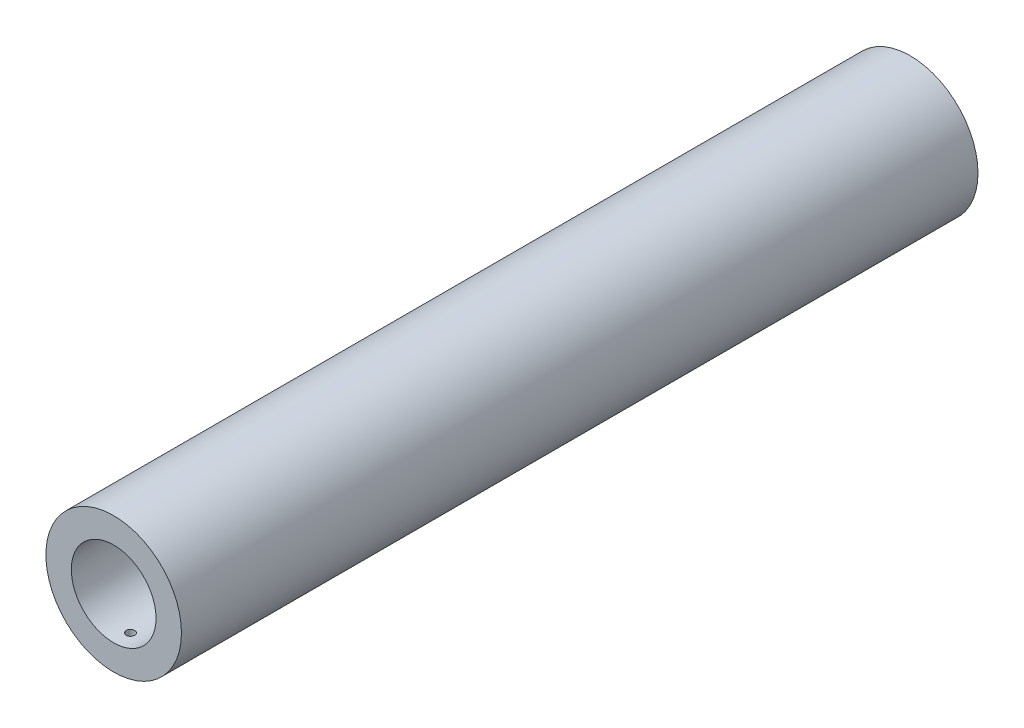
from build123d import *

# Parameters (mm, degrees)
SKETCH1_R               = 40
SKETCH1_R_2             = 25
BOSS_EXTRUDE1_DEPTH     = 470
CUT_EXTRUDE1_REACH      = 475.392
CUT_EXTRUDE1_END_RADIUS = 40
SKETCH2_R               = 2.5


with BuildPart() as part:
    # Sketch1 → Boss-Extrude1 (new body)
    with BuildSketch(Plane.XY):
        with Locations(Location((0, 0, 0), (0, 0, 180))):
            Circle(SKETCH1_R)
        with Locations(Location((0, 0, 0), (0, 0, 180))):
            Circle(SKETCH1_R_2, mode=Mode.SUBTRACT)
    extrude(amount=BOSS_EXTRUDE1_DEPTH)

    # Cut-Extrude1: up to this cylinder (the profile starts inside it)
    cut_extrude1_end = Plane(origin=(0, 0, 235), z_dir=(0, 0, -1)) * Cylinder(CUT_EXTRUDE1_END_RADIUS, 1481.784, mode=Mode.PRIVATE)
    # Sketch2 → Cut-Extrude1 (cut, up to the surface)
    with BuildSketch(Plane(origin=(0, 0, 0), x_dir=(1, 0, 0), z_dir=(0, 1, 0)), mode=Mode.PRIVATE) as cut_extrude1_sk1:
        with Locations(Location((0, -460, 0), (0, 0, 270))):
            Circle(SKETCH2_R)
    cut_extrude1_tool1 = extrude(cut_extrude1_sk1.sketch, amount=-CUT_EXTRUDE1_REACH, mode=Mode.PRIVATE) & cut_extrude1_end
    add(cut_extrude1_tool1.solids().sort_by_distance((0, 0, 460))[0], mode=Mode.SUBTRACT)
    # Sketch2 → Cut-Extrude1 (cut, up to the surface)
    with BuildSketch(Plane(origin=(0, 0, 0), x_dir=(1, 0, 0), z_dir=(0, 1, 0)), mode=Mode.PRIVATE) as cut_extrude1_sk2:
        with Locations(Location((0, -10, 0), (0, 0, 270))):
            Circle(SKETCH2_R)
    cut_extrude1_tool2 = extrude(cut_extrude1_sk2.sketch, amount=-CUT_EXTRUDE1_REACH, mode=Mode.PRIVATE) & cut_extrude1_end
    add(cut_extrude1_tool2.solids().sort_by_distance((0, 0, 10))[0], mode=Mode.SUBTRACT)


solid = part.part
